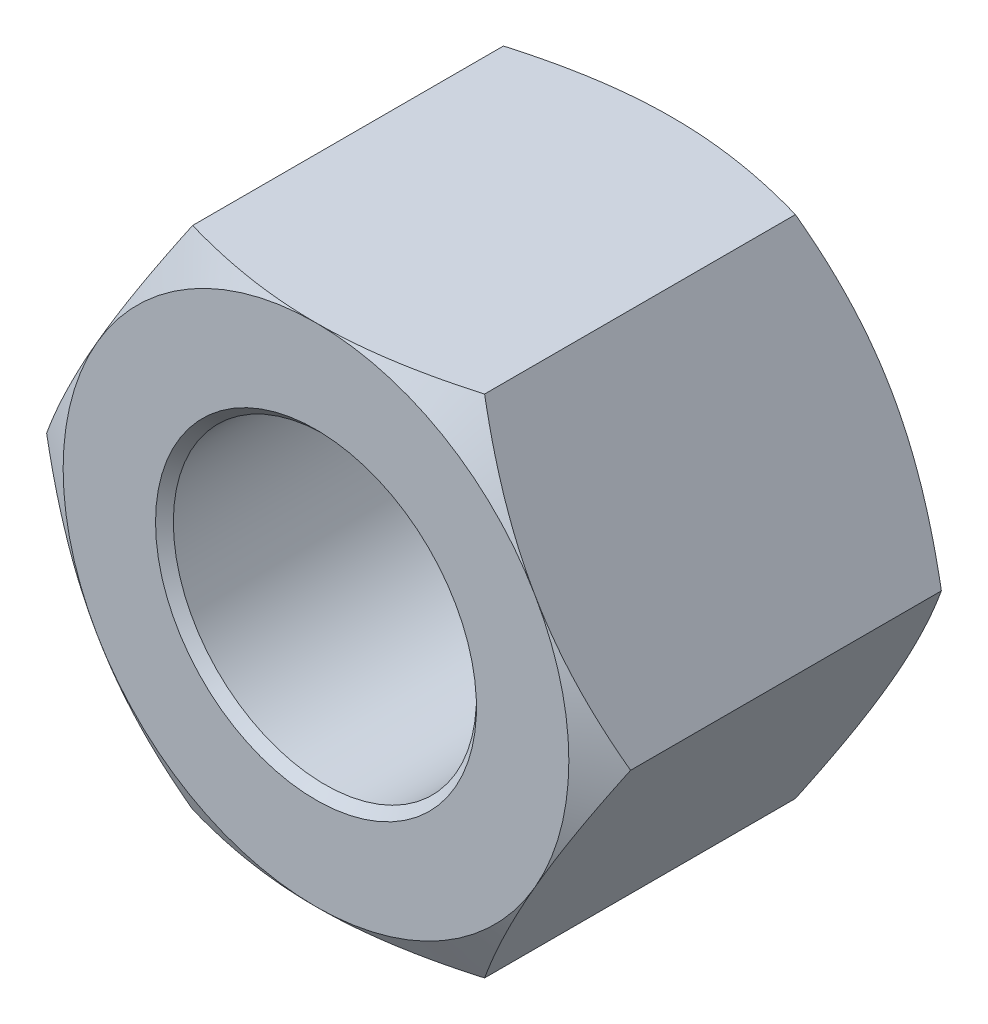
SolidWorks part; units mm, degrees
material "Steel"
ref_plane "Plane1" through (0, 0, 0) normal (0, 0, 1) x (1, 0, 0)
ref_plane "Plane2" through (0, 0, 0) normal (0, 1, 0) x (1, 0, 0)
ref_plane "Plane3" through (0, 0, 0) normal (1, 0, 0) x (0, 0, -1)
sketch "Dimension Sketch" plane through (0, 0, 0) normal (0, 0, 1) x (1, 0, 0)
  line L0 (0, 0) -> (21, 0) construction
  point P1 (19.2, 0)
  point P3 (14, 0)
  point P4 (2, 0)
  point P5 (22.8, 0)
  point P6 (13.9, 0)
  point P8 (21, 0)
  dimension "D" = 14
  dimension "e(最小)" = 22.8
  dimension "m(最大)" = 13.9
  dimension "s(公称)" = 21
  dimension "dw(最小)" = 19.2
  dimension "P" = 2
sketch "Sketch1" plane through (0, 0, 0) normal (0, 0, 1) x (1, 0, 0)
  line L0 (-26.8088, 0) -> (37.1748, 0) construction
  line L1 (0, 25.0215) -> (0, -25.0215) construction
  line L3 (5.7, 9.8727) -> (-5.7, 9.8727)
  line L4 (-5.7, 9.8727) -> (-11.4, 0)
  line L5 (-11.4, 0) -> (-5.7, -9.8727)
  line L6 (-5.7, -9.8727) -> (5.7, -9.8727)
  line L7 (5.7, -9.8727) -> (11.4, 0)
  line L8 (11.4, 0) -> (5.7, 9.8727)
  circle A0 centre (0, 0) radius 9.8727 construction
  circle A1 centre (0, 0) radius 5.9175
  dimension "D" = 11.835
  dimension "e" = 22.8
extrude "Boss-Extrude" add sketch "Sketch1" along normal blind 13.9
cosmetic thread "Cosmetic Thread1" parameters "D2"=14
sketch "Sketch2" plane through (0, 0, 0) normal (0, 0, -1) x (-1, 0, 0)
  line L0 (-5.7, 9.8727) -> (5.7, 9.8727) construction
  circle A0 centre (0, 0) radius 9.8727
  circle A1 centre (0, 0) radius 5.9175 construction
extrude "Cut-Extrude1" cut sketch "Sketch2" against normal through all draft 60 flip side to cut
sketch "Sketch3" plane through (0, 0, 13.9) normal (0, 0, 1) x (1, 0, 0)
  line L0 (11.4, 0) -> (5.7, 9.8727) construction
  circle A0 centre (0, 0) radius 9.8727
extrude "Cut-Extrude2" cut sketch "Sketch3" against normal through all draft 60 flip side to cut
chamfer "Chamfer1" distance 0.3475 angle 45 2 edges at (5.9175, 0, 0) (5.9175, 0, 13.9)
